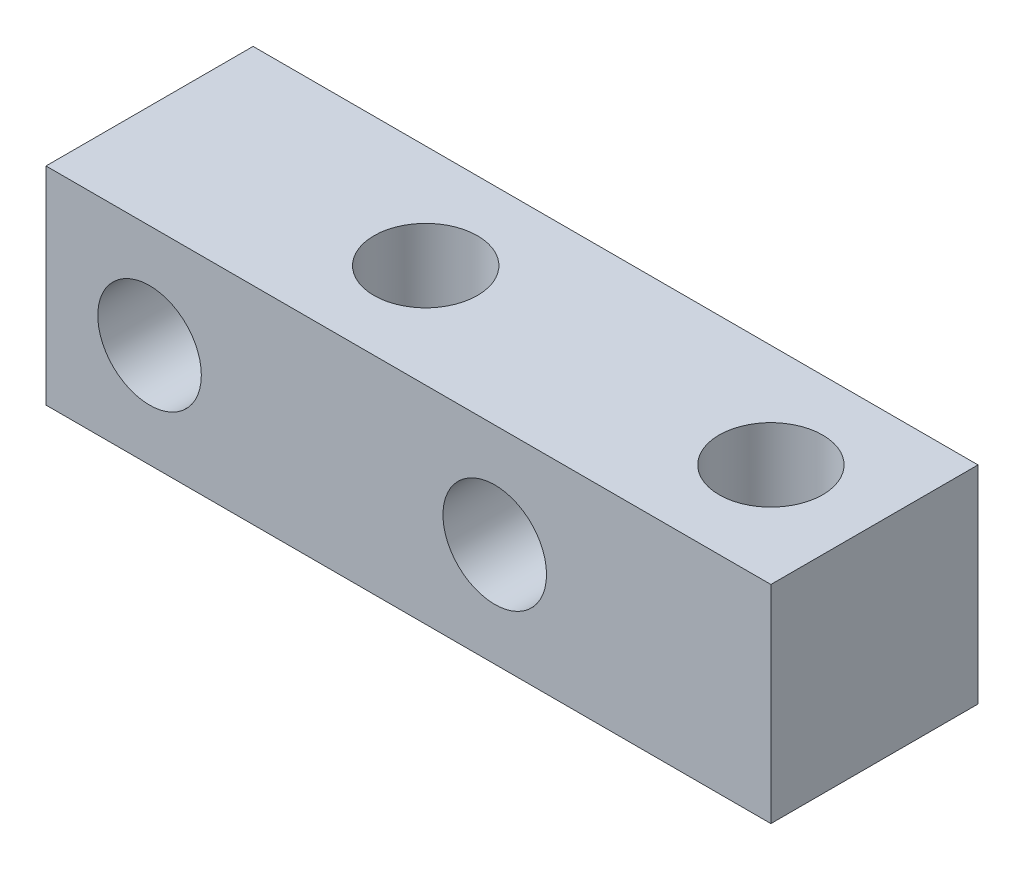
SolidWorks part; units mm, degrees
material "6061 合金"
ref_plane "前视基准面" through (0, 0, 0) normal (0, 0, 1) x (1, 0, 0)
ref_plane "上视基准面" through (0, 0, 0) normal (0, 1, 0) x (1, 0, 0)
ref_plane "右视基准面" through (0, 0, 0) normal (1, 0, 0) x (0, 0, -1)
other "Configuration Table"
sketch "草图1" plane through (0, 0, 0) normal (0, 0, 1) x (1, 0, 0)
  line L1 (0, 0) -> (21, 0)
  line L2 (0, 0) -> (0, 6)
  line L3 (0, 6) -> (21, 6)
  line L4 (21, 0) -> (21, 6)
  circle A0 centre (3, 3) radius 1.5
  circle A1 centre (13, 3) radius 1.5
  point P9 (0, 0)
  dimension "D3" = 3
  dimension "D5" = 3
  dimension "D6" = 10
  dimension "D1" = 6
  dimension "D2" = 21
  dimension "D4" = 3
extrude "凸台-拉伸1" add sketch "草图1" along normal blind 6
sketch "草图2" plane through (0, 6, 0) normal (0, 1, 0) x (1, 0, 0)
  line L0 (21, -6) -> (0, -6) construction
  line L1 (21, -6) -> (21, 0) construction
  circle A0 centre (8, -3) radius 1.5
  circle A1 centre (18, -3) radius 1.5
  point P4 (0, 0)
  dimension "D1" = 3
  dimension "D2" = 3
  dimension "D3" = 3
  dimension "D4" = 10
extrude "切除-拉伸1" cut sketch "草图2" against normal through all both and the other way through all
